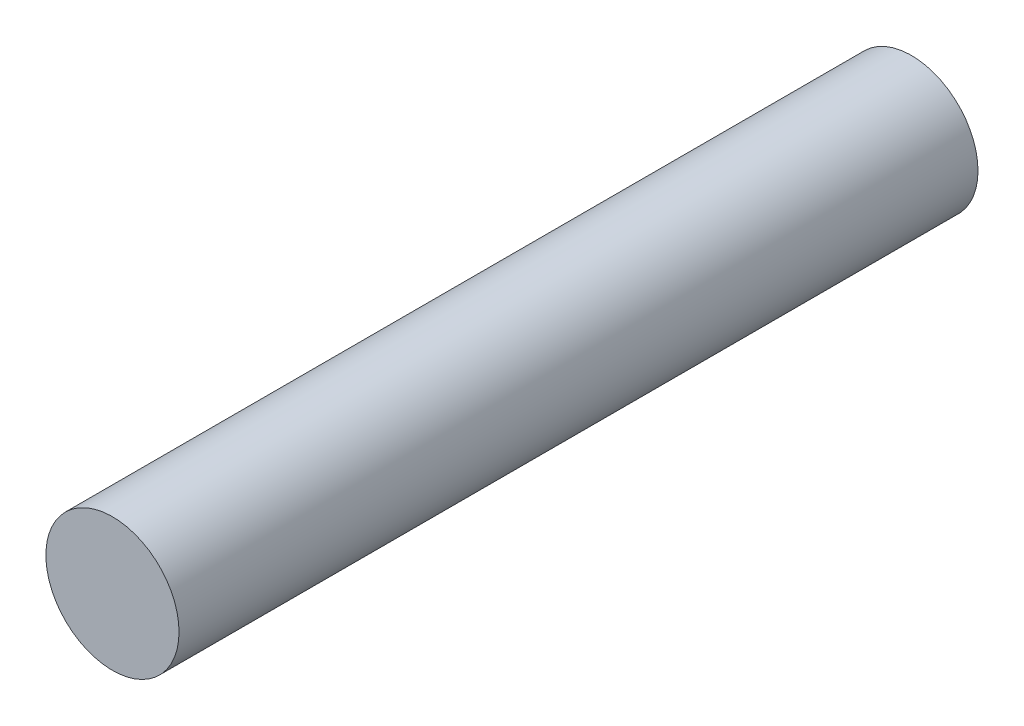
SolidWorks part; units mm, degrees
ref_plane "Front Plane" through (0, 0, 0) normal (0, 0, 1) x (1, 0, 0)
ref_plane "Top Plane" through (0, 0, 0) normal (0, 1, 0) x (1, 0, 0)
ref_plane "Right Plane" through (0, 0, 0) normal (1, 0, 0) x (0, 0, -1)
sketch "Sketch1" plane through (0, 0, 0) normal (0, 0, 1) x (1, 0, 0)
  circle A0 centre (0, 0) radius 100
  dimension "D1" = 200
extrude "Boss-Extrude1" add sketch "Sketch1" along normal blind 1200
